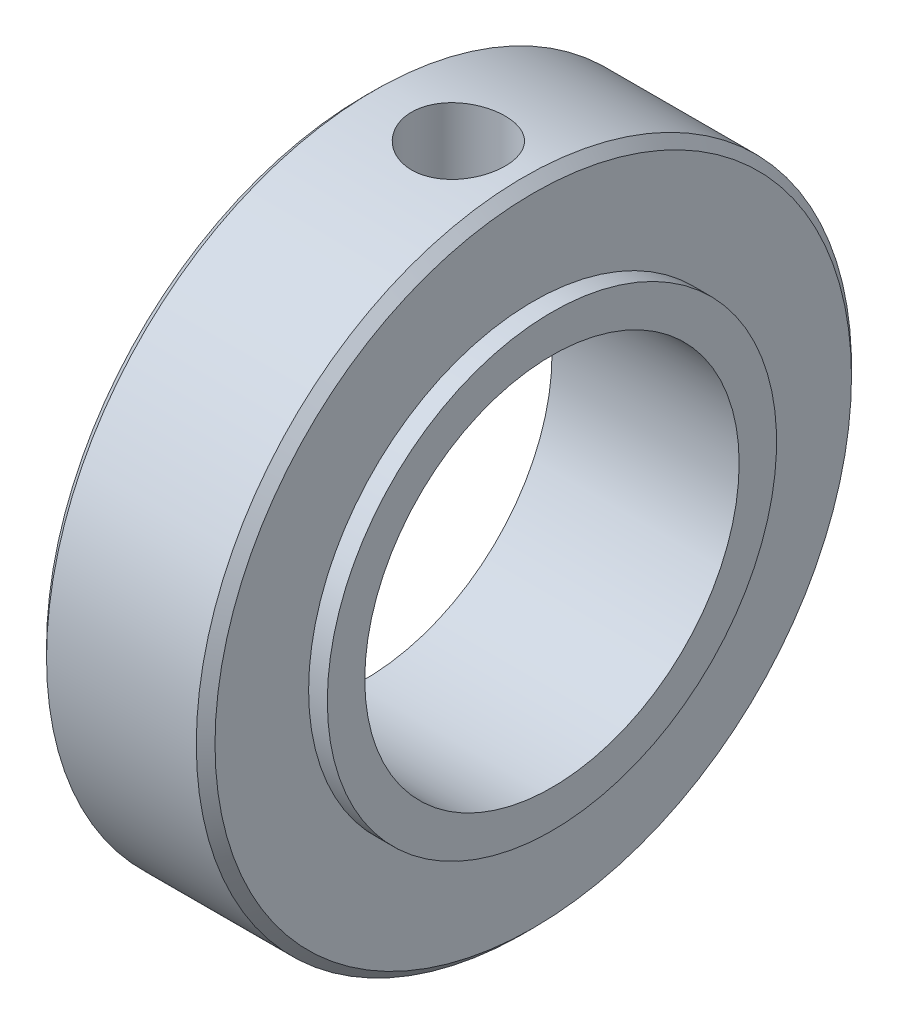
from build123d import *

# Parameters (mm, degrees)
M6_TAPPED_HOLE1_D               = 5
M6_TAPPED_HOLE1_DEPTH           = 15
M6_TAPPED_HOLE1_TIP             = 1.502151548
M6_TAPPED_HOLE1_ON_FACE_2_D     = 5
M6_TAPPED_HOLE1_ON_FACE_2_DEPTH = 15
M6_TAPPED_HOLE1_ON_FACE_2_TIP   = 1.502151548
CHAMFER1_SIZE                   = 0.5


with BuildPart() as part:
    # Sketch1 → Revolve1 (revolve)
    with BuildSketch(Plane.XY, mode=Mode.PRIVATE) as revolve1_sk:
        Polygon((0, 10), (10, 10), (10, 12), (9, 12), (9, 17.5), (0, 17.5), align=None)
    revolve(revolve1_sk.sketch.rotate(Axis((0, 0, 0), (1, 0, 0)), 90), axis=Axis((0, 0, 0), (1, 0, 0)))

    # M6 Tapped Hole1
    with Locations(Plane(origin=(5, 17.5, 0), x_dir=(0, 0, 1), z_dir=(0, 1, 0))):
        with Locations((0, 0)):
            Hole(M6_TAPPED_HOLE1_D / 2, depth=M6_TAPPED_HOLE1_DEPTH)
            with Locations((0, 0, -(M6_TAPPED_HOLE1_DEPTH + M6_TAPPED_HOLE1_TIP / 2))):  # 118° drill point
                Cone(0, M6_TAPPED_HOLE1_D / 2, M6_TAPPED_HOLE1_TIP, mode=Mode.SUBTRACT)

    # M6 Tapped Hole1 on face 2
    with Locations(Plane(origin=(-19.39268328, -13.895465991, 0), x_dir=(0, 0, 1), z_dir=(0, 1, 0))):
        with Locations((0, 0)):
            Hole(M6_TAPPED_HOLE1_ON_FACE_2_D / 2, depth=M6_TAPPED_HOLE1_ON_FACE_2_DEPTH)
            with Locations((0, 0, -(M6_TAPPED_HOLE1_ON_FACE_2_DEPTH + M6_TAPPED_HOLE1_ON_FACE_2_TIP / 2))):  # 118° drill point
                Cone(0, M6_TAPPED_HOLE1_ON_FACE_2_D / 2, M6_TAPPED_HOLE1_ON_FACE_2_TIP, mode=Mode.SUBTRACT)

    # Chamfer1
    chamfer1_edges = [part.edges().sort_by_distance(p)[0] for p in [
        (9, 0, -17.5),
        (0, 0, -17.5),
    ]]
    chamfer(chamfer1_edges, length=CHAMFER1_SIZE)


solid = part.part
